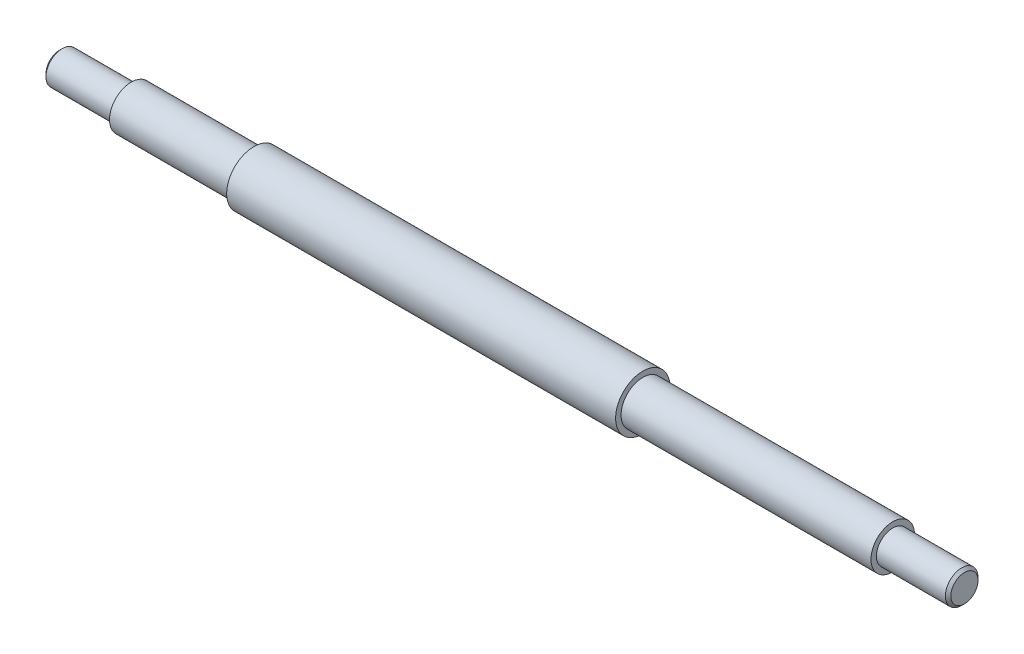
from build123d import *


with BuildPart() as part:
    # Model → Revolve1 (revolve)
    with BuildSketch(Plane.XY, mode=Mode.PRIVATE) as revolve1_sk:
        Polygon((-193.071714982, -28.205353865), (-193.071714982, -27.205353865), (-170.52661738, -27.205353865), (-170.52661738, -26.205353865), (-99.022420086, -26.205353865), (-99.022420086, -27.205353865), (-53.071714982, -27.205353865), (-53.071714982, -28.205353865), (-41.671714982, -28.205353865), (-40.394954521, -28.205353865), (-39.894954521, -28.705353865), (-39.894954521, -31.205353865), (-206.248475443, -31.205353865), (-206.248475443, -28.705353865), (-205.748475443, -28.205353865), (-199.071714982, -28.205353865), align=None)
    revolve(revolve1_sk.sketch.rotate(Axis((-206.248475443, -31.205353865, 0), (-1, 0, 0)), 90), axis=Axis((-206.248475443, -31.205353865, 0), (-1, 0, 0)))


solid = part.part
